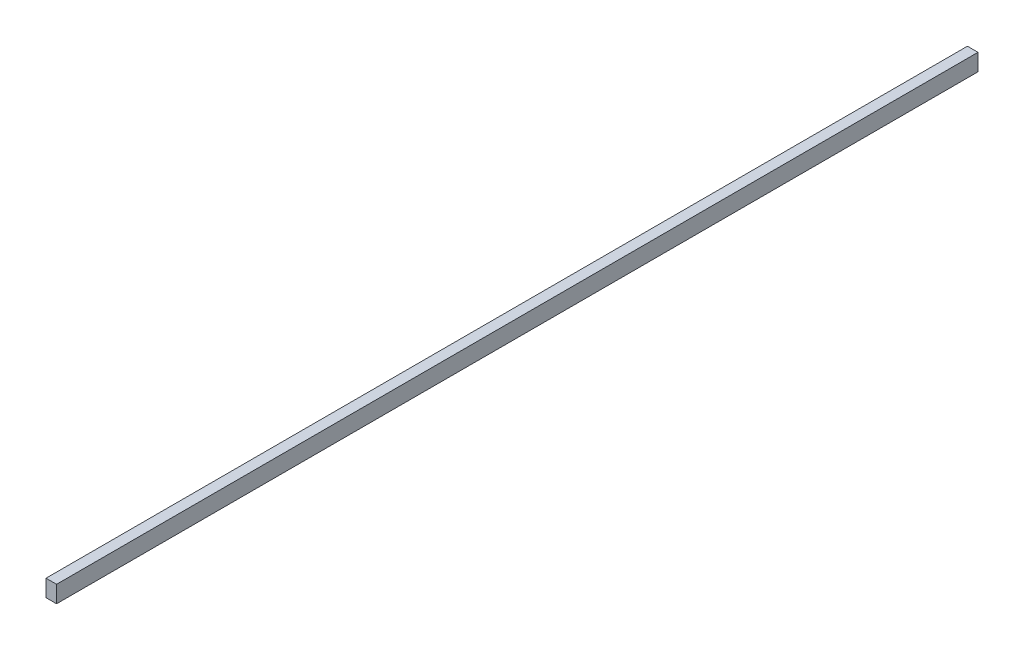
SolidWorks part; units mm, degrees
ref_plane "前视基准面" through (0, 0, 0) normal (0, 0, 1) x (1, 0, 0)
ref_plane "上视基准面" through (0, 0, 0) normal (0, 1, 0) x (1, 0, 0)
ref_plane "右视基准面" through (0, 0, 0) normal (1, 0, 0) x (0, 0, -1)
other "Configuration Table"
sketch "草图1" plane through (0, 0, 0) normal (0, 0, 1) x (1, 0, 0)
  line L0 (-448, 20) -> (-85, 20) construction
  line L1 (-85, 20) -> (-110, 20)
  line L2 (-85, 20) -> (-85, -20)
  line L3 (-85, -20) -> (-110, -20)
  line L4 (-110, 20) -> (-110, -20)
  line L6 (-85, -20) -> (-85, 20)
  line L7 (-85, 20) -> (-448, 20)
  line L8 (-448, 20) -> (-448, -20)
  line L9 (-448, -20) -> (-85, -20)
  line L10 (-85, -20) -> (-85, 20)
  line L13 (-85, 20) -> (-448, 20) construction
  line L14 (-448, 20) -> (-448, -20) construction
  line L15 (-448, -20) -> (-85, -20) construction
  dimension "D2" = 25
  dimension "D1" = 0
extrude "凸台-拉伸1" add sketch "草图1" along normal up to surface (2180.9801 mm away) contours L1 L4 L3 L2
